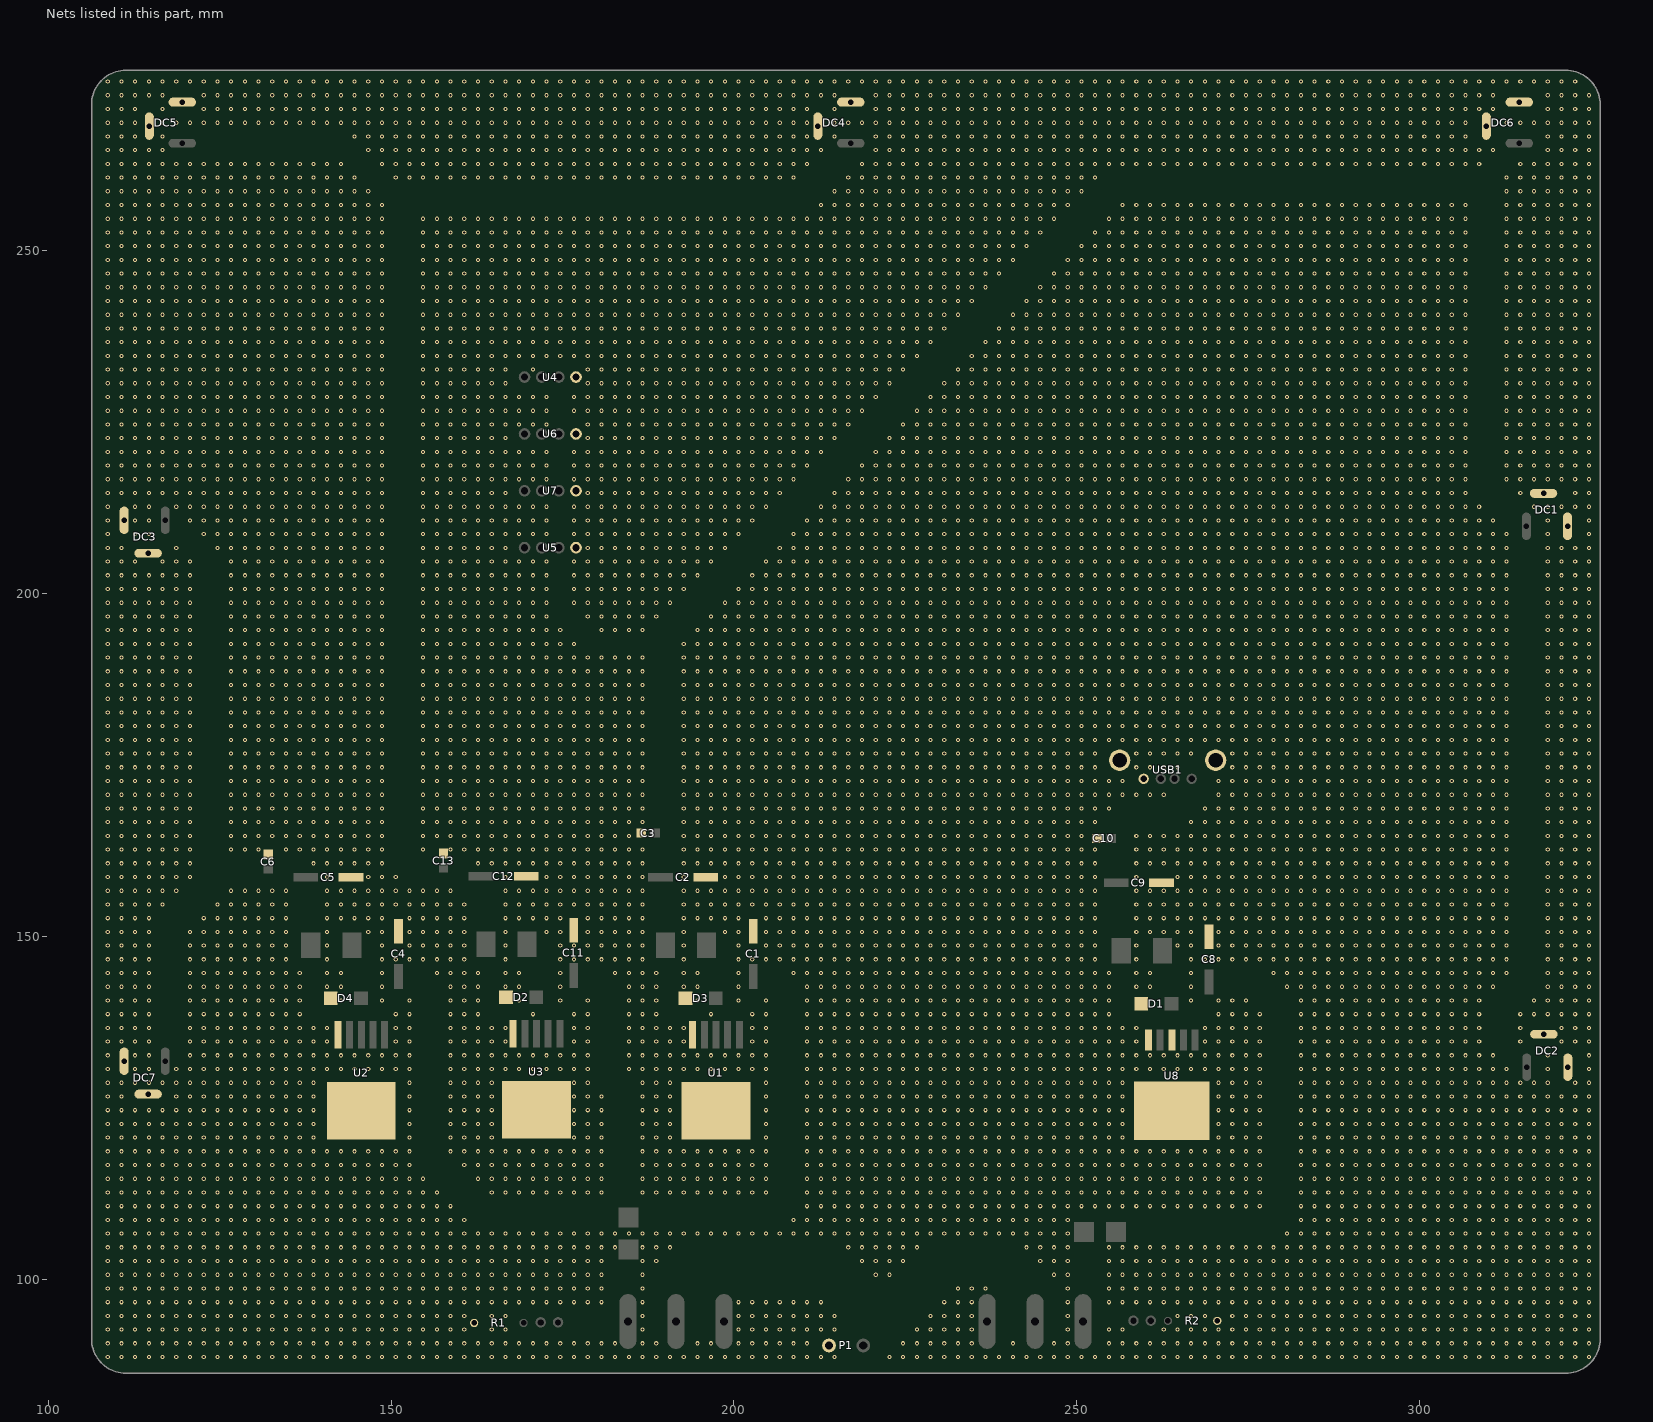
[diagram p0: the nets of this part, all layers, seen from the top]
# Altium PCB MISC49942.pcbdoc (part 2 of 4)
Units mm, origin at the board's own origin, x right, y up, seen from the top; angles counter-clockwise.
Board outline 220 x 190 mm, 2 copper layers (Top Layer, Bottom Layer), stack 1.58 mm thick; 45 components, 14 nets, 127 pads, 8689 vias.

## Via types
v1: diameter 0.61, hole 0.305, Top Layer to Bottom Layer, 8689 vias

## Nets (pads, with @x,y where several pads share a name; then routed paths per layer and width w, separated by ;. In a path a pad name is that pad's centre, name@x,y a point inside that pad or via, vN(x,y) a via of type N, cw(c..) or ccw(c..) an arc to the next point about the centre after c; other vN are vias at no path point) (continued)
GND: (continued)
  other v1: 108.684,88.669 110.684,88.669 112.684,88.669 114.684,88.669 116.684,88.669 118.684,88.669 120.684,88.669 122.684,88.669 124.684,88.669 126.684,88.669 128.684,88.669 130.684,88.669 132.684,88.669 134.684,88.669 136.684,88.669 138.684,88.669 140.684,88.669 142.684,88.669 144.684,88.669 146.684,88.669 148.684,88.669 150.684,88.669 152.684,88.669 154.684,88.669 156.684,88.669 158.684,88.669 160.684,88.669 162.684,88.669 164.684,88.669 166.684,88.669 168.684,88.669 170.684,88.669 172.684,88.669 174.684,88.669 176.684,88.669 178.684,88.669 180.684,88.669 182.684,88.669 184.684,88.669 186.684,88.669 188.684,88.669 190.684,88.669 192.684,88.669 194.684,88.669 196.684,88.669 198.684,88.669 200.684,88.669 202.684,88.669 204.684,88.669 206.684,88.669 208.684,88.669 210.684,88.669 212.684,88.669 214.684,88.669 222.684,88.669 224.684,88.669 226.684,88.669 228.684,88.669 230.684,88.669 232.684,88.669 234.684,88.669 236.684,88.669 238.684,88.669 240.684,88.669 242.684,88.669 244.684,88.669 246.684,88.669 248.684,88.669 250.684,88.669 252.684,88.669 254.684,88.669 256.684,88.669 258.684,88.669 260.684,88.669 262.684,88.669 264.684,88.669 266.684,88.669 268.684,88.669 270.684,88.669 272.684,88.669 274.684,88.669 276.684,88.669 278.684,88.669 280.684,88.669 282.684,88.669 284.684,88.669 286.684,88.669 288.684,88.669 290.684,88.669 292.684,88.669 294.684,88.669 296.684,88.669 298.684,88.669 300.684,88.669 302.684,88.669 304.684,88.669 306.684,88.669 308.684,88.669 310.684,88.669 312.684,88.669 314.684,88.669 316.684,88.669 318.684,88.669 320.684,88.669 322.684,88.669 324.684,88.669 108.684,90.669 110.684,90.669 112.684,90.669 114.684,90.669 116.684,90.669 118.684,90.669 120.684,90.669 122.684,90.669 124.684,90.669 126.684,90.669 128.684,90.669 130.684,90.669 132.684,90.669 134.684,90.669 136.684,90.669 138.684,90.669 140.684,90.669 142.684,90.669 144.684,90.669 146.684,90.669 148.684,90.669 150.684,90.669 152.684,90.669 154.684,90.669 156.684,90.669 158.684,90.669 160.684,90.669 162.684,90.669 164.684,90.669 166.684,90.669 168.684,90.669 170.684,90.669 172.684,90.669 174.684,90.669 176.684,90.669 178.684,90.669 180.684,90.669 182.684,90.669 186.684,90.669 188.684,90.669 194.684,90.669 196.684,90.669 200.684,90.669 202.684,90.669 204.684,90.669 206.684,90.669 208.684,90.669 210.684,90.669 224.684,90.669 226.684,90.669 228.684,90.669 230.684,90.669 232.684,90.669 234.684,90.669 240.684,90.669 246.684,90.669 248.684,90.669 254.684,90.669 256.684,90.669 258.684,90.669 260.684,90.669 262.684,90.669 264.684,90.669 266.684,90.669 268.684,90.669 270.684,90.669 272.684,90.669 274.684,90.669 276.684,90.669 278.684,90.669 280.684,90.669 282.684,90.669 284.684,90.669 286.684,90.669 288.684,90.669 290.684,90.669 292.684,90.669 294.684,90.669 296.684,90.669 298.684,90.669 300.684,90.669 302.684,90.669 304.684,90.669 306.684,90.669 308.684,90.669 310.684,90.669 312.684,90.669 314.684,90.669 316.684,90.669 318.684,90.669 320.684,90.669 322.684,90.669 324.684,90.669 108.684,92.669 110.684,92.669 112.684,92.669 114.684,92.669 116.684,92.669 118.684,92.669 120.684,92.669 122.684,92.669 124.684,92.669 126.684,92.669 128.684,92.669 130.684,92.669 132.684,92.669 134.684,92.669 136.684,92.669 138.684,92.669 140.684,92.669 142.684,92.669 144.684,92.669 146.684,92.669 148.684,92.669 150.684,92.669 152.684,92.669 154.684,92.669 156.684,92.669 158.684,92.669 160.684,92.669 164.684,92.669 166.684,92.669 186.684,92.669 200.684,92.669 202.684,92.669 204.684,92.669 206.684,92.669 208.684,92.669 210.684,92.669 212.684,92.669 214.684,92.669 226.684,92.669 228.684,92.669 230.684,92.669 232.684,92.669 234.684,92.669 248.684,92.669 254.684,92.669 256.684,92.669 262.684,92.669 264.684,92.669 266.684,92.669 268.684,92.669 270.684,92.669 272.684,92.669 274.684,92.669 276.684,92.669 278.684,92.669 280.684,92.669 282.684,92.669 284.684,92.669 286.684,92.669 288.684,92.669 290.684,92.669 292.684,92.669 294.684,92.669 296.684,92.669 298.684,92.669 300.684,92.669 302.684,92.669 304.684,92.669 306.684,92.669 308.684,92.669 310.684,92.669 312.684,92.669 314.684,92.669 316.684,92.669 318.684,92.669 320.684,92.669 322.684,92.669 324.684,92.669 108.684,94.669 110.684,94.669 112.684,94.669 114.684,94.669 116.684,94.669 118.684,94.669 120.684,94.669 122.684,94.669 124.684,94.669 126.684,94.669 128.684,94.669 130.684,94.669 132.684,94.669 134.684,94.669 136.684,94.669 138.684,94.669 140.684,94.669 142.684,94.669 144.684,94.669 146.684,94.669 148.684,94.669 150.684,94.669 152.684,94.669 154.684,94.669 156.684,94.669 158.684,94.669 160.684,94.669 164.684,94.669 166.684,94.669 186.684,94.669 200.684,94.669 202.684,94.669 204.684,94.669 206.684,94.669 208.684,94.669 210.684,94.669 212.684,94.669 214.684,94.669 228.684,94.669 230.684,94.669 232.684,94.669 234.684,94.669 248.684,94.669 264.684,94.669 266.684,94.669 268.684,94.669 272.684,94.669 274.684,94.669 276.684,94.669 278.684,94.669 280.684,94.669 282.684,94.669 284.684,94.669 286.684,94.669 288.684,94.669 290.684,94.669 292.684,94.669 294.684,94.669 296.684,94.669 298.684,94.669 300.684,94.669 302.684,94.669 304.684,94.669 306.684,94.669 308.684,94.669 310.684,94.669 312.684,94.669 314.684,94.669 316.684,94.669 318.684,94.669 320.684,94.669 322.684,94.669 324.684,94.669 108.684,96.669 110.684,96.669 112.684,96.669 114.684,96.669 116.684,96.669 118.684,96.669 120.684,96.669 122.684,96.669 124.684,96.669 126.684,96.669 128.684,96.669 130.684,96.669 132.684,96.669 134.684,96.669 136.684,96.669 138.684,96.669 140.684,96.669 142.684,96.669 144.684,96.669 146.684,96.669 148.684,96.669 150.684,96.669 152.684,96.669 154.684,96.669 156.684,96.669 158.684,96.669 160.684,96.669 162.684,96.669 164.684,96.669 166.684,96.669 168.684,96.669 170.684,96.669 172.684,96.669 174.684,96.669 176.684,96.669 178.684,96.669 180.684,96.669 186.684,96.669 200.684,96.669 202.684,96.669 204.684,96.669 206.684,96.669 208.684,96.669 210.684,96.669 212.684,96.669 230.684,96.669 232.684,96.669 234.684,96.669 248.684,96.669 254.684,96.669 256.684,96.669 258.684,96.669 260.684,96.669 262.684,96.669 264.684,96.669 266.684,96.669 268.684,96.669 270.684,96.669 272.684,96.669 274.684,96.669 276.684,96.669 278.684,96.669 280.684,96.669 282.684,96.669 284.684,96.669 286.684,96.669 288.684,96.669 290.684,96.669 292.684,96.669 294.684,96.669 296.684,96.669 298.684,96.669 300.684,96.669 302.684,96.669 304.684,96.669 306.684,96.669 308.684,96.669 310.684,96.669 312.684,96.669 314.684,96.669 316.684,96.669 318.684,96.669 320.684,96.669 322.684,96.669 324.684,96.669 108.684,98.669 110.684,98.669 112.684,98.669 114.684,98.669 116.684,98.669 118.684,98.669 120.684,98.669 122.684,98.669 124.684,98.669 126.684,98.669 128.684,98.669 130.684,98.669 132.684,98.669 134.684,98.669 136.684,98.669 138.684,98.669 140.684,98.669 142.684,98.669 144.684,98.669 146.684,98.669 148.684,98.669 150.684,98.669 152.684,98.669 154.684,98.669 156.684,98.669 158.684,98.669 160.684,98.669 162.684,98.669 164.684,98.669 166.684,98.669 168.684,98.669 170.684,98.669 172.684,98.669 174.684,98.669 176.684,98.669 178.684,98.669 180.684,98.669 186.684,98.669 232.684,98.669 234.684,98.669 236.684,98.669 248.684,98.669 254.684,98.669 256.684,98.669 258.684,98.669 260.684,98.669 262.684,98.669 264.684,98.669 266.684,98.669 268.684,98.669 270.684,98.669 272.684,98.669 274.684,98.669 276.684,98.669 278.684,98.669 280.684,98.669 282.684,98.669 284.684,98.669 286.684,98.669 288.684,98.669 290.684,98.669 292.684,98.669 294.684,98.669 296.684,98.669 298.684,98.669 300.684,98.669 302.684,98.669 304.684,98.669 306.684,98.669 308.684,98.669 310.684,98.669 312.684,98.669 314.684,98.669 316.684,98.669 318.684,98.669 320.684,98.669 322.684,98.669 324.684,98.669 108.684,100.669 110.684,100.669 112.684,100.669 114.684,100.669 116.684,100.669 118.684,100.669 120.684,100.669 122.684,100.669 124.684,100.669 126.684,100.669 128.684,100.669 130.684,100.669 132.684,100.669 134.684,100.669 136.684,100.669 138.684,100.669 140.684,100.669 142.684,100.669 144.684,100.669 146.684,100.669 148.684,100.669 150.684,100.669 152.684,100.669 154.684,100.669 156.684,100.669 158.684,100.669 160.684,100.669 162.684,100.669 164.684,100.669 166.684,100.669 168.684,100.669 170.684,100.669 172.684,100.669 174.684,100.669 176.684,100.669 178.684,100.669 180.684,100.669 186.684,100.669 220.684,100.669 222.684,100.669 246.684,100.669 248.684,100.669 254.684,100.669 256.684,100.669 258.684,100.669 260.684,100.669 262.684,100.669 264.684,100.669 266.684,100.669 268.684,100.669 270.684,100.669 272.684,100.669 274.684,100.669 276.684,100.669 278.684,100.669 280.684,100.669 282.684,100.669 284.684,100.669 286.684,100.669 288.684,100.669 290.684,100.669 292.684,100.669 294.684,100.669 296.684,100.669 298.684,100.669 300.684,100.669 302.684,100.669 304.684,100.669 306.684,100.669 308.684,100.669 310.684,100.669 312.684,100.669 314.684,100.669 316.684,100.669 318.684,100.669 320.684,100.669 322.684,100.669 324.684,100.669 108.684,102.669 110.684,102.669 112.684,102.669 114.684,102.669 116.684,102.669 118.684,102.669 120.684,102.669 122.684,102.669 124.684,102.669 126.684,102.669 128.684,102.669 130.684,102.669 132.684,102.669 134.684,102.669 136.684,102.669 138.684,102.669 140.684,102.669 142.684,102.669 144.684,102.669 146.684,102.669 148.684,102.669 150.684,102.669 152.684,102.669 154.684,102.669 156.684,102.669 158.684,102.669 160.684,102.669 162.684,102.669 164.684,102.669 166.684,102.669 168.684,102.669 170.684,102.669 172.684,102.669 174.684,102.669 176.684,102.669 178.684,102.669 180.684,102.669 186.684,102.669 188.684,102.669 218.684,102.669 220.684,102.669 222.684,102.669 224.684,102.669 244.684,102.669 246.684,102.669 248.684,102.669 254.684,102.669 256.684,102.669 258.684,102.669 260.684,102.669 262.684,102.669 264.684,102.669 266.684,102.669 268.684,102.669 270.684,102.669 272.684,102.669 274.684,102.669 276.684,102.669 278.684,102.669 280.684,102.669 282.684,102.669 284.684,102.669 286.684,102.669 288.684,102.669 290.684,102.669 292.684,102.669 294.684,102.669 296.684,102.669 298.684,102.669 300.684,102.669 302.684,102.669 304.684,102.669 306.684,102.669 308.684,102.669 310.684,102.669 312.684,102.669 314.684,102.669 316.684,102.669 318.684,102.669 320.684,102.669 322.684,102.669 324.684,102.669 108.684,104.669 110.684,104.669 112.684,104.669 114.684,104.669 116.684,104.669 118.684,104.669 120.684,104.669 122.684,104.669 124.684,104.669 126.684,104.669 128.684,104.669 130.684,104.669 132.684,104.669 134.684,104.669 136.684,104.669 138.684,104.669 140.684,104.669 142.684,104.669 144.684,104.669 146.684,104.669 148.684,104.669 150.684,104.669 152.684,104.669 154.684,104.669 156.684,104.669 158.684,104.669 160.684,104.669 162.684,104.669 164.684,104.669 166.684,104.669 168.684,104.669 170.684,104.669 172.684,104.669 174.684,104.669 176.684,104.669 178.684,104.669 180.684,104.669 182.684,104.669 186.684,104.669 188.684,104.669 190.684,104.669 216.684,104.669 218.684,104.669 220.684,104.669 222.684,104.669 224.684,104.669 226.684,104.669 242.684,104.669 244.684,104.669 246.684,104.669 248.684,104.669 254.684,104.669 256.684,104.669 258.684,104.669 260.684,104.669 262.684,104.669 264.684,104.669 266.684,104.669 268.684,104.669 270.684,104.669 272.684,104.669 274.684,104.669 276.684,104.669 278.684,104.669 280.684,104.669 282.684,104.669 284.684,104.669 286.684,104.669 288.684,104.669 290.684,104.669 292.684,104.669 294.684,104.669 296.684,104.669 298.684,104.669 300.684,104.669 302.684,104.669 304.684,104.669 306.684,104.669 308.684,104.669 310.684,104.669 312.684,104.669 314.684,104.669 316.684,104.669 318.684,104.669 320.684,104.669 322.684,104.669 324.684,104.669 108.684,106.669 110.684,106.669 112.684,106.669 114.684,106.669 116.684,106.669 118.684,106.669 120.684,106.669 122.684,106.669 124.684,106.669 126.684,106.669 128.684,106.669 130.684,106.669 132.684,106.669 134.684,106.669 136.684,106.669 138.684,106.669 140.684,106.669 142.684,106.669 144.684,106.669 146.684,106.669 148.684,106.669 150.684,106.669 152.684,106.669 154.684,106.669 156.684,106.669 158.684,106.669 160.684,106.669 162.684,106.669 164.684,106.669 166.684,106.669 168.684,106.669 170.684,106.669 172.684,106.669 174.684,106.669 176.684,106.669 178.684,106.669 180.684,106.669 182.684,106.669 184.684,106.669 186.684,106.669 188.684,106.669 190.684,106.669 192.684,106.669 194.684,106.669 196.684,106.669 198.684,106.669 200.684,106.669 202.684,106.669 204.684,106.669 206.684,106.669 208.684,106.669 210.684,106.669 212.684,106.669 214.684,106.669 216.684,106.669 218.684,106.669 220.684,106.669 222.684,106.669 224.684,106.669 226.684,106.669 228.684,106.669 230.684,106.669 232.684,106.669 234.684,106.669 236.684,106.669 238.684,106.669 240.684,106.669 242.684,106.669 244.684,106.669 246.684,106.669 248.684,106.669 280.684,106.669 282.684,106.669 284.684,106.669 286.684,106.669 288.684,106.669 290.684,106.669 292.684,106.669 294.684,106.669 296.684,106.669 298.684,106.669 300.684,106.669 302.684,106.669 304.684,106.669 306.684,106.669 308.684,106.669 310.684,106.669 312.684,106.669 314.684,106.669 316.684,106.669 318.684,106.669 320.684,106.669 322.684,106.669 324.684,106.669 108.684,108.669 110.684,108.669 112.684,108.669 114.684,108.669 116.684,108.669 118.684,108.669 120.684,108.669 122.684,108.669 124.684,108.669 126.684,108.669 128.684,108.669 130.684,108.669 132.684,108.669 134.684,108.669 136.684,108.669 138.684,108.669 140.684,108.669 142.684,108.669 144.684,108.669 146.684,108.669 148.684,108.669 150.684,108.669 152.684,108.669 154.684,108.669 156.684,108.669 158.684,108.669 160.684,108.669 208.684,108.669 210.684,108.669 212.684,108.669 214.684,108.669 216.684,108.669 218.684,108.669 220.684,108.669 222.684,108.669 224.684,108.669 226.684,108.669 228.684,108.669 230.684,108.669 232.684,108.669 234.684,108.669 236.684,108.669 238.684,108.669 240.684,108.669 242.684,108.669 244.684,108.669 246.684,108.669 248.684,108.669 282.684,108.669 284.684,108.669 286.684,108.669 288.684,108.669 290.684,108.669 292.684,108.669 294.684,108.669 296.684,108.669 298.684,108.669 300.684,108.669 302.684,108.669 304.684,108.669 306.684,108.669 308.684,108.669 310.684,108.669 312.684,108.669 314.684,108.669 316.684,108.669 318.684,108.669 320.684,108.669 322.684,108.669 324.684,108.669 108.684,110.669 110.684,110.669 112.684,110.669 114.684,110.669 116.684,110.669 118.684,110.669 120.684,110.669 122.684,110.669 124.684,110.669 126.684,110.669 128.684,110.669 130.684,110.669 132.684,110.669 134.684,110.669 136.684,110.669 138.684,110.669 140.684,110.669 142.684,110.669 144.684,110.669 146.684,110.669 148.684,110.669 150.684,110.669 152.684,110.669 154.684,110.669 156.684,110.669 158.684,110.669 210.684,110.669 212.684,110.669 214.684,110.669 216.684,110.669 218.684,110.669 220.684,110.669 222.684,110.669 224.684,110.669 226.684,110.669 228.684,110.669 230.684,110.669 232.684,110.669 234.684,110.669 236.684,110.669 238.684,110.669 240.684,110.669 242.684,110.669 244.684,110.669 246.684,110.669 248.684,110.669 250.684,110.669 252.684,110.669 254.684,110.669 256.684,110.669 258.684,110.669 260.684,110.669 262.684,110.669 264.684,110.669 266.684,110.669 268.684,110.669 270.684,110.669 272.684,110.669 274.684,110.669 276.684,110.669 282.684,110.669 284.684,110.669 286.684,110.669 288.684,110.669 290.684,110.669 292.684,110.669 294.684,110.669 296.684,110.669 298.684,110.669 300.684,110.669 302.684,110.669 304.684,110.669 306.684,110.669 308.684,110.669 310.684,110.669 312.684,110.669 314.684,110.669 316.684,110.669 318.684,110.669 320.684,110.669 322.684,110.669 324.684,110.669 108.684,112.669 110.684,112.669 112.684,112.669 114.684,112.669 116.684,112.669 118.684,112.669 120.684,112.669 122.684,112.669 124.684,112.669 126.684,112.669 128.684,112.669 130.684,112.669 132.684,112.669 134.684,112.669 136.684,112.669 138.684,112.669 140.684,112.669 142.684,112.669 144.684,112.669 146.684,112.669 148.684,112.669 150.684,112.669 152.684,112.669 154.684,112.669 156.684,112.669 164.684,112.669 166.684,112.669 168.684,112.669 170.684,112.669 172.684,112.669 174.684,112.669 176.684,112.669 178.684,112.669 180.684,112.669 186.684,112.669 188.684,112.669 190.684,112.669 192.684,112.669 194.684,112.669 196.684,112.669 198.684,112.669 200.684,112.669 202.684,112.669 204.684,112.669 210.684,112.669 212.684,112.669 214.684,112.669 216.684,112.669 218.684,112.669 220.684,112.669 222.684,112.669 224.684,112.669 226.684,112.669 228.684,112.669 230.684,112.669 232.684,112.669 234.684,112.669 236.684,112.669 238.684,112.669 240.684,112.669 242.684,112.669 244.684,112.669 246.684,112.669 248.684,112.669 250.684,112.669 252.684,112.669 254.684,112.669 256.684,112.669 258.684,112.669 260.684,112.669 262.684,112.669 264.684,112.669 266.684,112.669 268.684,112.669 270.684,112.669 272.684,112.669 274.684,112.669 276.684,112.669 282.684,112.669 284.684,112.669 286.684,112.669 288.684,112.669 290.684,112.669 292.684,112.669 294.684,112.669 296.684,112.669 298.684,112.669 300.684,112.669 302.684,112.669 304.684,112.669 306.684,112.669 308.684,112.669 310.684,112.669 312.684,112.669 314.684,112.669 316.684,112.669 318.684,112.669 320.684,112.669 322.684,112.669 324.684,112.669 108.684,114.669 110.684,114.669 112.684,114.669 114.684,114.669 116.684,114.669 118.684,114.669 120.684,114.669 122.684,114.669 124.684,114.669 126.684,114.669 128.684,114.669 130.684,114.669 132.684,114.669 134.684,114.669 136.684,114.669 138.684,114.669 140.684,114.669 142.684,114.669 144.684,114.669 146.684,114.669 148.684,114.669 150.684,114.669 152.684,114.669 154.684,114.669 162.684,114.669 164.684,114.669 166.684,114.669 168.684,114.669 170.684,114.669 172.684,114.669 174.684,114.669 176.684,114.669 178.684,114.669 180.684,114.669 186.684,114.669 188.684,114.669 190.684,114.669 192.684,114.669 194.684,114.669 196.684,114.669 198.684,114.669 200.684,114.669 202.684,114.669 204.684,114.669 210.684,114.669 212.684,114.669 214.684,114.669 216.684,114.669 218.684,114.669 220.684,114.669 222.684,114.669 224.684,114.669 226.684,114.669 228.684,114.669 230.684,114.669 232.684,114.669 234.684,114.669 236.684,114.669 238.684,114.669 240.684,114.669 242.684,114.669 244.684,114.669 246.684,114.669 248.684,114.669 250.684,114.669 252.684,114.669 254.684,114.669 256.684,114.669 258.684,114.669 260.684,114.669 262.684,114.669 264.684,114.669 266.684,114.669 268.684,114.669 270.684,114.669 272.684,114.669 274.684,114.669 276.684,114.669 282.684,114.669 284.684,114.669 286.684,114.669 288.684,114.669 290.684,114.669 292.684,114.669 294.684,114.669 296.684,114.669 298.684,114.669 300.684,114.669 302.684,114.669 304.684,114.669 306.684,114.669 308.684,114.669 310.684,114.669 312.684,114.669 314.684,114.669 316.684,114.669 318.684,114.669 320.684,114.669 322.684,114.669 324.684,114.669 108.684,116.669 110.684,116.669 112.684,116.669 114.684,116.669 116.684,116.669 118.684,116.669 120.684,116.669 122.684,116.669 124.684,116.669 126.684,116.669 128.684,116.669 130.684,116.669 132.684,116.669 134.684,116.669 136.684,116.669 138.684,116.669 140.684,116.669 142.684,116.669 144.684,116.669 146.684,116.669 148.684,116.669 150.684,116.669 152.684,116.669 160.684,116.669 162.684,116.669 164.684,116.669 166.684,116.669 168.684,116.669 170.684,116.669 172.684,116.669 174.684,116.669 176.684,116.669 178.684,116.669 180.684,116.669 186.684,116.669 188.684,116.669 190.684,116.669 192.684,116.669 194.684,116.669 196.684,116.669 198.684,116.669 200.684,116.669 202.684,116.669 204.684,116.669 210.684,116.669 212.684,116.669 214.684,116.669 216.684,116.669 218.684,116.669 220.684,116.669 222.684,116.669 224.684,116.669 226.684,116.669 228.684,116.669 230.684,116.669 232.684,116.669 234.684,116.669 236.684,116.669 238.684,116.669 240.684,116.669 242.684,116.669 244.684,116.669 246.684,116.669 248.684,116.669 250.684,116.669 252.684,116.669 254.684,116.669 256.684,116.669 258.684,116.669 260.684,116.669 262.684,116.669 264.684,116.669 266.684,116.669 268.684,116.669 270.684,116.669 272.684,116.669 274.684,116.669 276.684,116.669 282.684,116.669 284.684,116.669 286.684,116.669 288.684,116.669 290.684,116.669 292.684,116.669 294.684,116.669 296.684,116.669 298.684,116.669 300.684,116.669 302.684,116.669 304.684,116.669 306.684,116.669 308.684,116.669 310.684,116.669 312.684,116.669 314.684,116.669 316.684,116.669 318.684,116.669 320.684,116.669 322.684,116.669 324.684,116.669 108.684,118.669 110.684,118.669 112.684,118.669 114.684,118.669 116.684,118.669 118.684,118.669 120.684,118.669 122.684,118.669 124.684,118.669 126.684,118.669 128.684,118.669 130.684,118.669 132.684,118.669 134.684,118.669 136.684,118.669 138.684,118.669 140.684,118.669 142.684,118.669 144.684,118.669 146.684,118.669 148.684,118.669 150.684,118.669 152.684,118.669 158.684,118.669 160.684,118.669 162.684,118.669 164.684,118.669 166.684,118.669 168.684,118.669 170.684,118.669 172.684,118.669 174.684,118.669 176.684,118.669 178.684,118.669 180.684,118.669 186.684,118.669 188.684,118.669 190.684,118.669 192.684,118.669 194.684,118.669 196.684,118.669 198.684,118.669 200.684,118.669 202.684,118.669 204.684,118.669 210.684,118.669 212.684,118.669 214.684,118.669 216.684,118.669 218.684,118.669 220.684,118.669 222.684,118.669 224.684,118.669 226.684,118.669 228.684,118.669 230.684,118.669 232.684,118.669 234.684,118.669 236.684,118.669 238.684,118.669 240.684,118.669 242.684,118.669 244.684,118.669 246.684,118.669 248.684,118.669 250.684,118.669 252.684,118.669 254.684,118.669 256.684,118.669 258.684,118.669 260.684,118.669 262.684,118.669 264.684,118.669 266.684,118.669 268.684,118.669 270.684,118.669 272.684,118.669 274.684,118.669 276.684,118.669 282.684,118.669 284.684,118.669 286.684,118.669 288.684,118.669 290.684,118.669 292.684,118.669 294.684,118.669 296.684,118.669 298.684,118.669 300.684,118.669 302.684,118.669 304.684,118.669 306.684,118.669 308.684,118.669 310.684,118.669 312.684,118.669 314.684,118.669 316.684,118.669 318.684,118.669 320.684,118.669 322.684,118.669 324.684,118.669 108.684,120.669 110.684,120.669 112.684,120.669 114.684,120.669 116.684,120.669 118.684,120.669 120.684,120.669 122.684,120.669 124.684,120.669 126.684,120.669 128.684,120.669 130.684,120.669 132.684,120.669 134.684,120.669 136.684,120.669 138.684,120.669 152.684,120.669 158.684,120.669 160.684,120.669 162.684,120.669 164.684,120.669 176.684,120.669 178.684,120.669 180.684,120.669 186.684,120.669 188.684,120.669 190.684,120.669 204.684,120.669 210.684,120.669 212.684,120.669 214.684,120.669 216.684,120.669 218.684,120.669 220.684,120.669 222.684,120.669 224.684,120.669 226.684,120.669 228.684,120.669 230.684,120.669 232.684,120.669 234.684,120.669 236.684,120.669 238.684,120.669 240.684,120.669 242.684,120.669 244.684,120.669 246.684,120.669 248.684,120.669 250.684,120.669 252.684,120.669 254.684,120.669 256.684,120.669 270.684,120.669 272.684,120.669 274.684,120.669 276.684,120.669 282.684,120.669 284.684,120.669 286.684,120.669 288.684,120.669 290.684,120.669 292.684,120.669 294.684,120.669 296.684,120.669 298.684,120.669 300.684,120.669 302.684,120.669 304.684,120.669 306.684,120.669 308.684,120.669 310.684,120.669 312.684,120.669 314.684,120.669 316.684,120.669 318.684,120.669 320.684,120.669 322.684,120.669 324.684,120.669 108.684,122.669 110.684,122.669 112.684,122.669 114.684,122.669 116.684,122.669 118.684,122.669 120.684,122.669 122.684,122.669 124.684,122.669 126.684,122.669 128.684,122.669 130.684,122.669 132.684,122.669 134.684,122.669 136.684,122.669 138.684,122.669 152.684,122.669 158.684,122.669 160.684,122.669 162.684,122.669 164.684,122.669 176.684,122.669 178.684,122.669 180.684,122.669 186.684,122.669 188.684,122.669 190.684,122.669 204.684,122.669 210.684,122.669 212.684,122.669 214.684,122.669 216.684,122.669 218.684,122.669 220.684,122.669 222.684,122.669 224.684,122.669 226.684,122.669 228.684,122.669 230.684,122.669 232.684,122.669 234.684,122.669 236.684,122.669 238.684,122.669 240.684,122.669 242.684,122.669 244.684,122.669 246.684,122.669 248.684,122.669 250.684,122.669 252.684,122.669 254.684,122.669 256.684,122.669 270.684,122.669 272.684,122.669 274.684,122.669 276.684,122.669 282.684,122.669 284.684,122.669 286.684,122.669 288.684,122.669 290.684,122.669 292.684,122.669 294.684,122.669 296.684,122.669 298.684,122.669 300.684,122.669 302.684,122.669 304.684,122.669 306.684,122.669 308.684,122.669 310.684,122.669 312.684,122.669 314.684,122.669 316.684,122.669 318.684,122.669 320.684,122.669 322.684,122.669 324.684,122.669 108.684,124.669 110.684,124.669 112.684,124.669 114.684,124.669 116.684,124.669 118.684,124.669 120.684,124.669 122.684,124.669 124.684,124.669 126.684,124.669 128.684,124.669 130.684,124.669 132.684,124.669 134.684,124.669 136.684,124.669 138.684,124.669 152.684,124.669 158.684,124.669 160.684,124.669 162.684,124.669 164.684,124.669 176.684,124.669 178.684,124.669 180.684,124.669 186.684,124.669 188.684,124.669 190.684,124.669 204.684,124.669 210.684,124.669 212.684,124.669 214.684,124.669 216.684,124.669 218.684,124.669 220.684,124.669 222.684,124.669 224.684,124.669 226.684,124.669 228.684,124.669 230.684,124.669 232.684,124.669 234.684,124.669 236.684,124.669 238.684,124.669 240.684,124.669 242.684,124.669 244.684,124.669 246.684,124.669 248.684,124.669 250.684,124.669 252.684,124.669 254.684,124.669 256.684,124.669 270.684,124.669 272.684,124.669 274.684,124.669 276.684,124.669 282.684,124.669 284.684,124.669 286.684,124.669 288.684,124.669 290.684,124.669 292.684,124.669 294.684,124.669 296.684,124.669 298.684,124.669 300.684,124.669 302.684,124.669 304.684,124.669 306.684,124.669 308.684,124.669 310.684,124.669 312.684,124.669 314.684,124.669 316.684,124.669 318.684,124.669 320.684,124.669 322.684,124.669 324.684,124.669 108.684,126.669 110.684,126.669 118.684,126.669 120.684,126.669 122.684,126.669 124.684,126.669 126.684,126.669 128.684,126.669 130.684,126.669 132.684,126.669 134.684,126.669 136.684,126.669 138.684,126.669 152.684,126.669 158.684,126.669 160.684,126.669 162.684,126.669 164.684,126.669 176.684,126.669 178.684,126.669 180.684,126.669 186.684,126.669 188.684,126.669 190.684,126.669 204.684,126.669 210.684,126.669 212.684,126.669 214.684,126.669 216.684,126.669 218.684,126.669 220.684,126.669 222.684,126.669 224.684,126.669 226.684,126.669 228.684,126.669 230.684,126.669 232.684,126.669 234.684,126.669 236.684,126.669 238.684,126.669 240.684,126.669 242.684,126.669 244.684,126.669 246.684,126.669 248.684,126.669 250.684,126.669 252.684,126.669 254.684,126.669 256.684,126.669 270.684,126.669 272.684,126.669 274.684,126.669 276.684,126.669 282.684,126.669 284.684,126.669 286.684,126.669 288.684,126.669 290.684,126.669 292.684,126.669 294.684,126.669 296.684,126.669 298.684,126.669 300.684,126.669 302.684,126.669 304.684,126.669 306.684,126.669 308.684,126.669 310.684,126.669 312.684,126.669 314.684,126.669 316.684,126.669 318.684,126.669 320.684,126.669 322.684,126.669 324.684,126.669 108.684,128.669 110.684,128.669 112.684,128.669 114.684,128.669 116.684,128.669 118.684,128.669 120.684,128.669 122.684,128.669 124.684,128.669 126.684,128.669 128.684,128.669 130.684,128.669 132.684,128.669 134.684,128.669 136.684,128.669 138.684,128.669 152.684,128.669 158.684,128.669 160.684,128.669 162.684,128.669 164.684,128.669 176.684,128.669 178.684,128.669 186.684,128.669 188.684,128.669 190.684,128.669 204.684,128.669 210.684,128.669 212.684,128.669 214.684,128.669 216.684,128.669 218.684,128.669 220.684,128.669 222.684,128.669 224.684,128.669 226.684,128.669 228.684,128.669 230.684,128.669 232.684,128.669 234.684,128.669 236.684,128.669 238.684,128.669 240.684,128.669 242.684,128.669 244.684,128.669 246.684,128.669 248.684,128.669 250.684,128.669 252.684,128.669 254.684,128.669 256.684,128.669 270.684,128.669 272.684,128.669 274.684,128.669 276.684,128.669 282.684,128.669 284.684,128.669 286.684,128.669 288.684,128.669 290.684,128.669 292.684,128.669 294.684,128.669 296.684,128.669 298.684,128.669 300.684,128.669 302.684,128.669 304.684,128.669 306.684,128.669 308.684,128.669 310.684,128.669 312.684,128.669 314.684,128.669 316.684,128.669 318.684,128.669 322.684,128.669 324.684,128.669 108.684,130.669 112.684,130.669 114.684,130.669 118.684,130.669 120.684,130.669 122.684,130.669 124.684,130.669 126.684,130.669 128.684,130.669 130.684,130.669 132.684,130.669 134.684,130.669 136.684,130.669 138.684,130.669 140.684,130.669 142.684,130.669 144.684,130.669 146.684,130.669 148.684,130.669 150.684,130.669 152.684,130.669 158.684,130.669 160.684,130.669 162.684,130.669 164.684,130.669 166.684,130.669 168.684,130.669 170.684,130.669 172.684,130.669 174.684,130.669 176.684,130.669 178.684,130.669 184.684,130.669 186.684,130.669 188.684,130.669 190.684,130.669 192.684,130.669 194.684,130.669 196.684,130.669 198.684,130.669 200.684,130.669 202.684,130.669 204.684,130.669 210.684,130.669 212.684,130.669 214.684,130.669 216.684,130.669 218.684,130.669 220.684,130.669 222.684,130.669 224.684,130.669 226.684,130.669 228.684,130.669 230.684,130.669 232.684,130.669 234.684,130.669 236.684,130.669 238.684,130.669 240.684,130.669 242.684,130.669 244.684,130.669 246.684,130.669 248.684,130.669 250.684,130.669 252.684,130.669 254.684,130.669 256.684,130.669 258.684,130.669 260.684,130.669 262.684,130.669 264.684,130.669 266.684,130.669 268.684,130.669 270.684,130.669 272.684,130.669 274.684,130.669 276.684,130.669 282.684,130.669 284.684,130.669 286.684,130.669 288.684,130.669 290.684,130.669 292.684,130.669 294.684,130.669 296.684,130.669 298.684,130.669 300.684,130.669 302.684,130.669 304.684,130.669 306.684,130.669 308.684,130.669 310.684,130.669 312.684,130.669 318.684,130.669 324.684,130.669 108.684,132.669 112.684,132.669 114.684,132.669 120.684,132.669 122.684,132.669 124.684,132.669 126.684,132.669 128.684,132.669 130.684,132.669 132.684,132.669 134.684,132.669 136.684,132.669 138.684,132.669 140.684,132.669 142.684,132.669 144.684,132.669 146.684,132.669 148.684,132.669 150.684,132.669 152.684,132.669 158.684,132.669 160.684,132.669 162.684,132.669 164.684,132.669 166.684,132.669 168.684,132.669 170.684,132.669 172.684,132.669 174.684,132.669 176.684,132.669 178.684,132.669 184.684,132.669 186.684,132.669 188.684,132.669 190.684,132.669 192.684,132.669 194.684,132.669 196.684,132.669 198.684,132.669 200.684,132.669 202.684,132.669 204.684,132.669 210.684,132.669 212.684,132.669 214.684,132.669 216.684,132.669 218.684,132.669 220.684,132.669 222.684,132.669 224.684,132.669 226.684,132.669 228.684,132.669 230.684,132.669 232.684,132.669 234.684,132.669 236.684,132.669 238.684,132.669 240.684,132.669 242.684,132.669 244.684,132.669 246.684,132.669 248.684,132.669 250.684,132.669 252.684,132.669 254.684,132.669 256.684,132.669 258.684,132.669 260.684,132.669 262.684,132.669 264.684,132.669 266.684,132.669 268.684,132.669 270.684,132.669 272.684,132.669 274.684,132.669 276.684,132.669 282.684,132.669 284.684,132.669 286.684,132.669 288.684,132.669 290.684,132.669 292.684,132.669 294.684,132.669 296.684,132.669 298.684,132.669 300.684,132.669 302.684,132.669 304.684,132.669 306.684,132.669 308.684,132.669 310.684,132.669 318.684,132.669 324.684,132.669 108.684,134.669 110.684,134.669 112.684,134.669 114.684,134.669 120.684,134.669 122.684,134.669 124.684,134.669 126.684,134.669 128.684,134.669 130.684,134.669 132.684,134.669 134.684,134.669 136.684,134.669 138.684,134.669 140.684,134.669 150.684,134.669 152.684,134.669 158.684,134.669 160.684,134.669 162.684,134.669 164.684,134.669 166.684,134.669 176.684,134.669 178.684,134.669 184.684,134.669 186.684,134.669 188.684,134.669 190.684,134.669 192.684,134.669 202.684,134.669 204.684,134.669 210.684,134.669 212.684,134.669 214.684,134.669 216.684,134.669 218.684,134.669 220.684,134.669 222.684,134.669 224.684,134.669 226.684,134.669 228.684,134.669 230.684,134.669 232.684,134.669 234.684,134.669 236.684,134.669 238.684,134.669 240.684,134.669 242.684,134.669 244.684,134.669 246.684,134.669 248.684,134.669 250.684,134.669 252.684,134.669 254.684,134.669 256.684,134.669 258.684,134.669 268.684,134.669 270.684,134.669 272.684,134.669 274.684,134.669 276.684,134.669 282.684,134.669 284.684,134.669 286.684,134.669 288.684,134.669 290.684,134.669 292.684,134.669 294.684,134.669 296.684,134.669 298.684,134.669 300.684,134.669 302.684,134.669 304.684,134.669 306.684,134.669 308.684,134.669 314.684,134.669 320.684,134.669 322.684,134.669 324.684,134.669 108.684,136.669 110.684,136.669 112.684,136.669 114.684,136.669 120.684,136.669 122.684,136.669 124.684,136.669 126.684,136.669 128.684,136.669 130.684,136.669 132.684,136.669 134.684,136.669 136.684,136.669 138.684,136.669 140.684,136.669 150.684,136.669 152.684,136.669 158.684,136.669 160.684,136.669 162.684,136.669 164.684,136.669 166.684,136.669 176.684,136.669 178.684,136.669 184.684,136.669 186.684,136.669 188.684,136.669 190.684,136.669 192.684,136.669 202.684,136.669 204.684,136.669 210.684,136.669 212.684,136.669 214.684,136.669 216.684,136.669 218.684,136.669 220.684,136.669 222.684,136.669 224.684,136.669 226.684,136.669 228.684,136.669 230.684,136.669 232.684,136.669 234.684,136.669 236.684,136.669 238.684,136.669 240.684,136.669 242.684,136.669 244.684,136.669 246.684,136.669 248.684,136.669 250.684,136.669 252.684,136.669 254.684,136.669 256.684,136.669 258.684,136.669 268.684,136.669 270.684,136.669 272.684,136.669 274.684,136.669 276.684,136.669 282.684,136.669 284.684,136.669 286.684,136.669 288.684,136.669 290.684,136.669 292.684,136.669 294.684,136.669 296.684,136.669 298.684,136.669 300.684,136.669 302.684,136.669 304.684,136.669 306.684,136.669 308.684,136.669 314.684,136.669 320.684,136.669 322.684,136.669 324.684,136.669 108.684,138.669 110.684,138.669 112.684,138.669 114.684,138.669 120.684,138.669 122.684,138.669 124.684,138.669 126.684,138.669 128.684,138.669 130.684,138.669 132.684,138.669 134.684,138.669 136.684,138.669 150.684,138.669 152.684,138.669 158.684,138.669 160.684,138.669 162.684,138.669 170.684,138.669 176.684,138.669 178.684,138.669 184.684,138.669 186.684,138.669 188.684,138.669 196.684,138.669 202.684,138.669 204.684,138.669 210.684,138.669 212.684,138.669 214.684,138.669 216.684,138.669 218.684,138.669 220.684,138.669 222.684,138.669 224.684,138.669 226.684,138.669 228.684,138.669 230.684,138.669 232.684,138.669 234.684,138.669 236.684,138.669 238.684,138.669 240.684,138.669 242.684,138.669 244.684,138.669 246.684,138.669 248.684,138.669 250.684,138.669 252.684,138.669 254.684,138.669 270.684,138.669 272.684,138.669 274.684,138.669 276.684,138.669 282.684,138.669 284.684,138.669 286.684,138.669 288.684,138.669 290.684,138.669 292.684,138.669 294.684,138.669 296.684,138.669 298.684,138.669 300.684,138.669 302.684,138.669 304.684,138.669 306.684,138.669 308.684,138.669 314.684,138.669 316.684,138.669 318.684,138.669 320.684,138.669 322.684,138.669 324.684,138.669 108.684,140.669 110.684,140.669 112.684,140.669 114.684,140.669 120.684,140.669 122.684,140.669 124.684,140.669 126.684,140.669 128.684,140.669 130.684,140.669 132.684,140.669 134.684,140.669 136.684,140.669 142.684,140.669 148.684,140.669 152.684,140.669 158.684,140.669 160.684,140.669 162.684,140.669 168.684,140.669 174.684,140.669 178.684,140.669 184.684,140.669 186.684,140.669 188.684,140.669 194.684,140.669 200.684,140.669 204.684,140.669 210.684,140.669 212.684,140.669 214.684,140.669 216.684,140.669 218.684,140.669 220.684,140.669 222.684,140.669 224.684,140.669 226.684,140.669 228.684,140.669 230.684,140.669 232.684,140.669 234.684,140.669 236.684,140.669 238.684,140.669 240.684,140.669 242.684,140.669 244.684,140.669 246.684,140.669 248.684,140.669 250.684,140.669 252.684,140.669 254.684,140.669 266.684,140.669 270.684,140.669 272.684,140.669 274.684,140.669 282.684,140.669 284.684,140.669 286.684,140.669 288.684,140.669 290.684,140.669 292.684,140.669 294.684,140.669 296.684,140.669 298.684,140.669 300.684,140.669 302.684,140.669 304.684,140.669 306.684,140.669 308.684,140.669 316.684,140.669 318.684,140.669 320.684,140.669 322.684,140.669 324.684,140.669 108.684,142.669 110.684,142.669 112.684,142.669 114.684,142.669 120.684,142.669 122.684,142.669 124.684,142.669 126.684,142.669 128.684,142.669 130.684,142.669 132.684,142.669 134.684,142.669 136.684,142.669 140.684,142.669 142.684,142.669 148.684,142.669 158.684,142.669 160.684,142.669 162.684,142.669 166.684,142.669 168.684,142.669 174.684,142.669 184.684,142.669 186.684,142.669 188.684,142.669 192.684,142.669 194.684,142.669 200.684,142.669 210.684,142.669 212.684,142.669 214.684,142.669 216.684,142.669 218.684,142.669 220.684,142.669 222.684,142.669 224.684,142.669 226.684,142.669 228.684,142.669 230.684,142.669 232.684,142.669 234.684,142.669 236.684,142.669 238.684,142.669 240.684,142.669 242.684,142.669 244.684,142.669 246.684,142.669 248.684,142.669 250.684,142.669 252.684,142.669 254.684,142.669 258.684,142.669 260.684,142.669 266.684,142.669 280.684,142.669 282.684,142.669 284.684,142.669 286.684,142.669 288.684,142.669 290.684,142.669 292.684,142.669 294.684,142.669 296.684,142.669 298.684,142.669 300.684,142.669 302.684,142.669 304.684,142.669 306.684,142.669 308.684,142.669 310.684,142.669 318.684,142.669 320.684,142.669 322.684,142.669 324.684,142.669 108.684,144.669 110.684,144.669 112.684,144.669 114.684,144.669 120.684,144.669 122.684,144.669 124.684,144.669 126.684,144.669 128.684,144.669 130.684,144.669 132.684,144.669 134.684,144.669 136.684,144.669 140.684,144.669 142.684,144.669 148.684,144.669 156.684,144.669 158.684,144.669 160.684,144.669 162.684,144.669 166.684,144.669 168.684,144.669 174.684,144.669 182.684,144.669 184.684,144.669 186.684,144.669 188.684,144.669 192.684,144.669 194.684,144.669 200.684,144.669 208.684,144.669 210.684,144.669 212.684,144.669 214.684,144.669 216.684,144.669 218.684,144.669 220.684,144.669 222.684,144.669 224.684,144.669 226.684,144.669 228.684,144.669 230.684,144.669 232.684,144.669 234.684,144.669 236.684,144.669 238.684,144.669 240.684,144.669 242.684,144.669 244.684,144.669 246.684,144.669 248.684,144.669 250.684,144.669 252.684,144.669 254.684,144.669 258.684,144.669 260.684,144.669 266.684,144.669 278.684,144.669 280.684,144.669 282.684,144.669 284.684,144.669 286.684,144.669 288.684,144.669 290.684,144.669 292.684,144.669 294.684,144.669 296.684,144.669 298.684,144.669 300.684,144.669 302.684,144.669 304.684,144.669 306.684,144.669 308.684,144.669 310.684,144.669 312.684,144.669 318.684,144.669 320.684,144.669 322.684,144.669 324.684,144.669 108.684,146.669 110.684,146.669 112.684,146.669 114.684,146.669 120.684,146.669 122.684,146.669 124.684,146.669 126.684,146.669 128.684,146.669 130.684,146.669 132.684,146.669 134.684,146.669 140.684,146.669 148.684,146.669 150.684,146.669 152.684,146.669 154.684,146.669 156.684,146.669 158.684,146.669 160.684,146.669 166.684,146.669 174.684,146.669 176.684,146.669 178.684,146.669 180.684,146.669 182.684,146.669 184.684,146.669 186.684,146.669 192.684,146.669 200.684,146.669 202.684,146.669 204.684,146.669 206.684,146.669 208.684,146.669 210.684,146.669 212.684,146.669 214.684,146.669 216.684,146.669 218.684,146.669 220.684,146.669 222.684,146.669 224.684,146.669 226.684,146.669 228.684,146.669 230.684,146.669 232.684,146.669 234.684,146.669 236.684,146.669 238.684,146.669 240.684,146.669 242.684,146.669 244.684,146.669 246.684,146.669 248.684,146.669 250.684,146.669 252.684,146.669 258.684,146.669 266.684,146.669 268.684,146.669 270.684,146.669 272.684,146.669 274.684,146.669 276.684,146.669 278.684,146.669 280.684,146.669 282.684,146.669 284.684,146.669 286.684,146.669 288.684,146.669 290.684,146.669 292.684,146.669 294.684,146.669 296.684,146.669 298.684,146.669 300.684,146.669 302.684,146.669 304.684,146.669 306.684,146.669 308.684,146.669 310.684,146.669 312.684,146.669 318.684,146.669 320.684,146.669 322.684,146.669 324.684,146.669 108.684,148.669 110.684,148.669 112.684,148.669 114.684,148.669 120.684,148.669 122.684,148.669 124.684,148.669 126.684,148.669 128.684,148.669 130.684,148.669 132.684,148.669 134.684,148.669 140.684,148.669 148.684,148.669 152.684,148.669 154.684,148.669 156.684,148.669 158.684,148.669 160.684,148.669 166.684,148.669 174.684,148.669 176.684,148.669 178.684,148.669 180.684,148.669 182.684,148.669 184.684,148.669 186.684,148.669 192.684,148.669 200.684,148.669 204.684,148.669 206.684,148.669 208.684,148.669 210.684,148.669 212.684,148.669 214.684,148.669 216.684,148.669 218.684,148.669 220.684,148.669 222.684,148.669 224.684,148.669 226.684,148.669 228.684,148.669 230.684,148.669 232.684,148.669 234.684,148.669 236.684,148.669 238.684,148.669 240.684,148.669 242.684,148.669 244.684,148.669 246.684,148.669 248.684,148.669 250.684,148.669 252.684,148.669 258.684,148.669 264.684,148.669 266.684,148.669 270.684,148.669 272.684,148.669 274.684,148.669 276.684,148.669 278.684,148.669 280.684,148.669 282.684,148.669 284.684,148.669 286.684,148.669 288.684,148.669 290.684,148.669 292.684,148.669 294.684,148.669 296.684,148.669 298.684,148.669 300.684,148.669 302.684,148.669 304.684,148.669 306.684,148.669 308.684,148.669 310.684,148.669 312.684,148.669 318.684,148.669 320.684,148.669 322.684,148.669 324.684,148.669 108.684,150.669 110.684,150.669 112.684,150.669 114.684,150.669 120.684,150.669 122.684,150.669 124.684,150.669 126.684,150.669 128.684,150.669 130.684,150.669 132.684,150.669 134.684,150.669 140.684,150.669 146.684,150.669 148.684,150.669 152.684,150.669 154.684,150.669 156.684,150.669 158.684,150.669 160.684,150.669 166.684,150.669 172.684,150.669 174.684,150.669 178.684,150.669 180.684,150.669 182.684,150.669 184.684,150.669 186.684,150.669 192.684,150.669 198.684,150.669 200.684,150.669 204.684,150.669 206.684,150.669 208.684,150.669 210.684,150.669 212.684,150.669 214.684,150.669 216.684,150.669 218.684,150.669 220.684,150.669 222.684,150.669 224.684,150.669 226.684,150.669 228.684,150.669 230.684,150.669 232.684,150.669 234.684,150.669 236.684,150.669 238.684,150.669 240.684,150.669 242.684,150.669 244.684,150.669 246.684,150.669 248.684,150.669 250.684,150.669 252.684,150.669 258.684,150.669 260.684,150.669 262.684,150.669 264.684,150.669 266.684,150.669 270.684,150.669 272.684,150.669 274.684,150.669 276.684,150.669 278.684,150.669 280.684,150.669 282.684,150.669 284.684,150.669 286.684,150.669 288.684,150.669 290.684,150.669 292.684,150.669 294.684,150.669 296.684,150.669 298.684,150.669 300.684,150.669 302.684,150.669 304.684,150.669 306.684,150.669 308.684,150.669 310.684,150.669 312.684,150.669 318.684,150.669 320.684,150.669 322.684,150.669 324.684,150.669 108.684,152.669 110.684,152.669 112.684,152.669 114.684,152.669 122.684,152.669 124.684,152.669 126.684,152.669 128.684,152.669 130.684,152.669 132.684,152.669 134.684,152.669 140.684,152.669 142.684,152.669 144.684,152.669 146.684,152.669 148.684,152.669 152.684,152.669 154.684,152.669 156.684,152.669 158.684,152.669 160.684,152.669 166.684,152.669 168.684,152.669 170.684,152.669 172.684,152.669 174.684,152.669 178.684,152.669 180.684,152.669 182.684,152.669 184.684,152.669 186.684,152.669 192.684,152.669 194.684,152.669 196.684,152.669 198.684,152.669 200.684,152.669 204.684,152.669 206.684,152.669 208.684,152.669 210.684,152.669 212.684,152.669 214.684,152.669 216.684,152.669 218.684,152.669 220.684,152.669 222.684,152.669 224.684,152.669 226.684,152.669 228.684,152.669 230.684,152.669 232.684,152.669 234.684,152.669 236.684,152.669 238.684,152.669 240.684,152.669 242.684,152.669 244.684,152.669 246.684,152.669 248.684,152.669 250.684,152.669 252.684,152.669 258.684,152.669 260.684,152.669 262.684,152.669 264.684,152.669 266.684,152.669 268.684,152.669 270.684,152.669 272.684,152.669 274.684,152.669 276.684,152.669 278.684,152.669 280.684,152.669 282.684,152.669 284.684,152.669 286.684,152.669 288.684,152.669 290.684,152.669 292.684,152.669 294.684,152.669 296.684,152.669 298.684,152.669 300.684,152.669 302.684,152.669 304.684,152.669 306.684,152.669 308.684,152.669 310.684,152.669 312.684,152.669 318.684,152.669 320.684,152.669 322.684,152.669 324.684,152.669 108.684,154.669 110.684,154.669 112.684,154.669 114.684,154.669 116.684,154.669 124.684,154.669 126.684,154.669 128.684,154.669 130.684,154.669 132.684,154.669 134.684,154.669 140.684,154.669 142.684,154.669 144.684,154.669 146.684,154.669 148.684,154.669 150.684,154.669 152.684,154.669 154.684,154.669 156.684,154.669 158.684,154.669 160.684,154.669 166.684,154.669 168.684,154.669 170.684,154.669 172.684,154.669 174.684,154.669 176.684,154.669 178.684,154.669 180.684,154.669 182.684,154.669 184.684,154.669 186.684,154.669 192.684,154.669 194.684,154.669 196.684,154.669 198.684,154.669 200.684,154.669 202.684,154.669 204.684,154.669 206.684,154.669 208.684,154.669 210.684,154.669 212.684,154.669 214.684,154.669 216.684,154.669 218.684,154.669 220.684,154.669 222.684,154.669 224.684,154.669 226.684,154.669 228.684,154.669 230.684,154.669 232.684,154.669 234.684,154.669 236.684,154.669 238.684,154.669 240.684,154.669 242.684,154.669 244.684,154.669 246.684,154.669 248.684,154.669 250.684,154.669 252.684,154.669 258.684,154.669 260.684,154.669 262.684,154.669 264.684,154.669 266.684,154.669 268.684,154.669 270.684,154.669 272.684,154.669 274.684,154.669 276.684,154.669 278.684,154.669 280.684,154.669 282.684,154.669 284.684,154.669 286.684,154.669 288.684,154.669 290.684,154.669 292.684,154.669 294.684,154.669 296.684,154.669 298.684,154.669 300.684,154.669 302.684,154.669 304.684,154.669 306.684,154.669 308.684,154.669 310.684,154.669 312.684,154.669 318.684,154.669 320.684,154.669 322.684,154.669 324.684,154.669 108.684,156.669 110.684,156.669 112.684,156.669 114.684,156.669 116.684,156.669 118.684,156.669 126.684,156.669 128.684,156.669 130.684,156.669 132.684,156.669 134.684,156.669 140.684,156.669 142.684,156.669 144.684,156.669 146.684,156.669 148.684,156.669 150.684,156.669 152.684,156.669 154.684,156.669 156.684,156.669 158.684,156.669 166.684,156.669 168.684,156.669 170.684,156.669 172.684,156.669 174.684,156.669 176.684,156.669 178.684,156.669 180.684,156.669 182.684,156.669 184.684,156.669 186.684,156.669 192.684,156.669 194.684,156.669 196.684,156.669 198.684,156.669 200.684,156.669 202.684,156.669 204.684,156.669 206.684,156.669 208.684,156.669 210.684,156.669 212.684,156.669 214.684,156.669 216.684,156.669 218.684,156.669 220.684,156.669 222.684,156.669 224.684,156.669 226.684,156.669 228.684,156.669 230.684,156.669 232.684,156.669 234.684,156.669 236.684,156.669 238.684,156.669 240.684,156.669 242.684,156.669 244.684,156.669 246.684,156.669 248.684,156.669 250.684,156.669 252.684,156.669 258.684,156.669 260.684,156.669 262.684,156.669 264.684,156.669 266.684,156.669 268.684,156.669 270.684,156.669 272.684,156.669 274.684,156.669 276.684,156.669 278.684,156.669 280.684,156.669 282.684,156.669 284.684,156.669 286.684,156.669 288.684,156.669 290.684,156.669 292.684,156.669 294.684,156.669 296.684,156.669 298.684,156.669 300.684,156.669 302.684,156.669 304.684,156.669 306.684,156.669 308.684,156.669 310.684,156.669 312.684,156.669 318.684,156.669 320.684,156.669 322.684,156.669 324.684,156.669 108.684,158.669 110.684,158.669 112.684,158.669 114.684,158.669 116.684,158.669 118.684,158.669 120.684,158.669 140.684,158.669 146.684,158.669 148.684,158.669 150.684,158.669 166.684,158.669 172.684,158.669 174.684,158.669 176.684,158.669 178.684,158.669 180.684,158.669 182.684,158.669 184.684,158.669 186.684,158.669 192.684,158.669 198.684,158.669 200.684,158.669 202.684,158.669 204.684,158.669 206.684,158.669 208.684,158.669 210.684,158.669 212.684,158.669 214.684,158.669 216.684,158.669 218.684,158.669 220.684,158.669 222.684,158.669 224.684,158.669 226.684,158.669 228.684,158.669 230.684,158.669 232.684,158.669 234.684,158.669 236.684,158.669 238.684,158.669 240.684,158.669 242.684,158.669 244.684,158.669 246.684,158.669 248.684,158.669 250.684,158.669 252.684,158.669 258.684,158.669 264.684,158.669 266.684,158.669 268.684,158.669